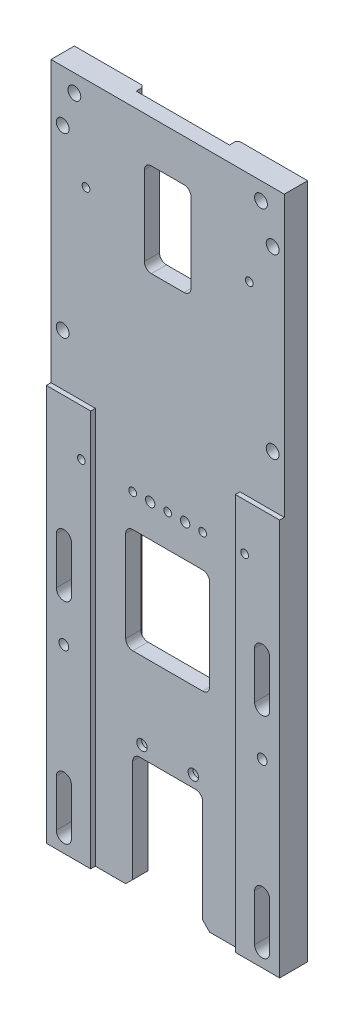
from build123d import *

# Parameters (mm, degrees)
SKETCH1_W                                            = 100
SKETCH1_H                                            = 290
BOSS_EXTRUDE1_DEPTH                                  = 10
SKETCH4_W                                            = 40
SKETCH4_H                                            = 290
CUT_EXTRUDE3_DEPTH                                   = 3.5
SKETCH5_R                                            = 2.75
CUT_EXTRUDE4_DEPTH                                   = 18
LPATTERN1_COUNT                                      = 2
LPATTERN1_PITCH                                      = 76
CUT_EXTRUDE5_DEPTH                                   = 18
LPATTERN2_COUNT                                      = 2
LPATTERN2_PITCH                                      = 90
SKETCH9_W                                            = 30
SKETCH9_H                                            = 50
CUT_EXTRUDE7_DEPTH                                   = 25
BOSS_EXTRUDE3_START                                  = 2
SKETCH11_W                                           = 19
SKETCH11_H                                           = 170
BOSS_EXTRUDE3_DEPTH                                  = 2
SKETCH12_R                                           = 2.75
CUT_EXTRUDE8_DEPTH                                   = 154.704261489
CHAMFER1_SIZE                                        = 3
FILLET1_R                                            = 3
SKETCH20_R                                           = 2
CUT_EXTRUDE14_DEPTH                                  = 10
M5_TAPPED_HOLE1_D                                    = 4.2
M4_TAPPED_HOLE2_D                                    = 3.3
F_4_0_4_DIAMETER_HOLE1_D                             = 4
CUT_EXTRUDE15_DEPTH                                  = 154.704261489
CHAMFER2_SIZE                                        = 1
HOLE_SIZE_PER_SOCKET_HEAD_CAP_SCREW_TYPE_D           = 4.5
HOLE_SIZE_PER_SOCKET_HEAD_CAP_SCREW_TYPE_CBORE_D     = 8
HOLE_SIZE_PER_SOCKET_HEAD_CAP_SCREW_TYPE_CBORE_DEPTH = 4.5
CUT_EXTRUDE16_DEPTH                                  = 154.847326919
M4_TAPPED_HOLE4_D                                    = 3.3


with BuildPart() as part:
    # Sketch1 → Boss-Extrude1 (new body)
    with BuildSketch(Plane.XY):
        Rectangle(SKETCH1_W, SKETCH1_H)
    extrude(amount=BOSS_EXTRUDE1_DEPTH)

    # Sketch4 → Cut-Extrude3 (cut)
    with BuildSketch(Plane(origin=(0, 0, 0), x_dir=(-1, 0, 0), z_dir=(0, 0, -1))):
        Rectangle(SKETCH4_W, SKETCH4_H)
    extrude(amount=-CUT_EXTRUDE3_DEPTH, mode=Mode.SUBTRACT)

    # Sketch5 → Cut-Extrude4 (cut)
    with BuildSketch(Plane.XY.offset(10)):
        with Locations((-45, 123)):
            Circle(SKETCH5_R)
        with Locations((45, 123)):
            Circle(SKETCH5_R)
    cut_extrude4 = extrude(amount=-CUT_EXTRUDE4_DEPTH, mode=Mode.SUBTRACT)

    # LPattern1: Cut-Extrude4 ×2
    with Locations(*[(0, -i * LPATTERN1_PITCH, 0) for i in range(1, LPATTERN1_COUNT)]):
        add(cut_extrude4, mode=Mode.SUBTRACT)

    # Sketch6 → Cut-Extrude5 (cut)
    with BuildSketch(Plane.XY.offset(10)):
        with BuildLine():
            Line((-39.25, -28), (-39.25, -48))
            ThreePointArc((-39.25, -48), (-42.5, -51.25), (-45.75, -48))
            Line((-45.75, -48), (-45.75, -28))
            ThreePointArc((-45.75, -28), (-42.5, -24.75), (-39.25, -28))
        make_face()
        with BuildLine():
            Line((39.25, -28), (39.25, -48))
            ThreePointArc((39.25, -48), (42.5, -51.25), (45.75, -48))
            Line((45.75, -48), (45.75, -28))
            ThreePointArc((45.75, -28), (42.5, -24.75), (39.25, -28))
        make_face()
    cut_extrude5 = extrude(amount=-CUT_EXTRUDE5_DEPTH, mode=Mode.SUBTRACT)

    # LPattern2: Cut-Extrude5 ×2
    with Locations(*[(0, -i * LPATTERN2_PITCH, 0) for i in range(1, LPATTERN2_COUNT)]):
        add(cut_extrude5, mode=Mode.SUBTRACT)

    # Sketch9 → Cut-Extrude7 (cut)
    with BuildSketch(Plane.XY.offset(10)):
        with Locations((0, -120)):
            Rectangle(SKETCH9_W, SKETCH9_H)
    extrude(amount=-CUT_EXTRUDE7_DEPTH, mode=Mode.SUBTRACT)

    # Sketch11 → Boss-Extrude3 (add)
    # profile 1 of 2: a face of its own
    with BuildSketch(Plane.XY.offset(10).offset(BOSS_EXTRUDE3_START)):
        with Locations((-40.5, -60)):
            Rectangle(SKETCH11_W, SKETCH11_H)
        with BuildLine():
            Line((-39.25, -138), (-39.25, -118))
            ThreePointArc((-39.25, -118), (-42.5, -114.75), (-45.75, -118))
            Line((-45.75, -118), (-45.75, -138))
            ThreePointArc((-45.75, -138), (-42.5, -141.25), (-39.25, -138))
        make_face(mode=Mode.SUBTRACT)
        with BuildLine():
            Line((-39.25, -48), (-39.25, -28))
            ThreePointArc((-39.25, -28), (-42.5, -24.75), (-45.75, -28))
            Line((-45.75, -28), (-45.75, -48))
            ThreePointArc((-45.75, -48), (-42.5, -51.25), (-39.25, -48))
        make_face(mode=Mode.SUBTRACT)
    # profile 2 of 2: a face of its own
    with BuildSketch(Plane.XY.offset(10).offset(BOSS_EXTRUDE3_START)):
        with Locations((40.5, -60)):
            Rectangle(SKETCH11_W, SKETCH11_H)
        with BuildLine():
            Line((45.75, -138), (45.75, -118))
            ThreePointArc((45.75, -118), (42.5, -114.75), (39.25, -118))
            Line((39.25, -118), (39.25, -138))
            ThreePointArc((39.25, -138), (42.5, -141.25), (45.75, -138))
        make_face(mode=Mode.SUBTRACT)
        with BuildLine():
            Line((45.75, -48), (45.75, -28))
            ThreePointArc((45.75, -28), (42.5, -24.75), (39.25, -28))
            Line((39.25, -28), (39.25, -48))
            ThreePointArc((39.25, -48), (42.5, -51.25), (45.75, -48))
        make_face(mode=Mode.SUBTRACT)
    extrude(amount=-BOSS_EXTRUDE3_DEPTH)

    # Sketch12 → Cut-Extrude8 (cut, through all)
    with BuildSketch(Plane.XY.offset(10)):
        with Locations((-40, 137.5)):
            Circle(SKETCH12_R)
        with Locations(Location((40, 137.5, 0), (0, 0, 180))):
            Circle(SKETCH12_R)
    extrude(amount=-CUT_EXTRUDE8_DEPTH, mode=Mode.SUBTRACT)

    # Chamfer1
    chamfer1_edges = [part.edges().sort_by_distance(p)[0] for p in [
        (15, -145, 6.75),
        (-15, -145, 6.75),
    ]]
    chamfer(chamfer1_edges, length=CHAMFER1_SIZE)

    # Fillet1
    fillet1_edges = [part.edges().sort_by_distance(p)[0] for p in [
        (15, -95, 6.75),
        (-15, -95, 6.75),
    ]]
    fillet(fillet1_edges, radius=FILLET1_R)

    # Sketch20 → Cut-Extrude14 (cut)
    with BuildSketch(Plane.XY.offset(12)):
        with Locations((-42.5, -67.5)):
            Circle(SKETCH20_R)
        with Locations(Location((42.5, -67.5, 0), (0, 0, 180))):
            Circle(SKETCH20_R)
    extrude(amount=-CUT_EXTRUDE14_DEPTH, mode=Mode.SUBTRACT)

    # M5 Tapped Hole1 (through all)
    with Locations(Plane(origin=(-42.5, -67.5, 12), x_dir=(1, 0, 0), z_dir=(0, 0, 1))):
        with Locations((0, 0), (85, 0)):
            Hole(M5_TAPPED_HOLE1_D / 2)

    # M4 Tapped Hole2 (through all)
    with Locations(Plane.XY.offset(10)):
        with Locations((-15, 2), (0, 2), (15, 2)):
            Hole(M4_TAPPED_HOLE2_D / 2)

    # Ø4.0 (4) Diameter Hole1 (through all)
    with Locations(Plane.XY.offset(10)):
        with Locations((-7.5, 2), (7.5, 2)):
            Hole(F_4_0_4_DIAMETER_HOLE1_D / 2)

    # Sketch26 → Cut-Extrude15 (cut, through all)
    with BuildSketch(Plane.XY.offset(10)):
        with BuildLine():
            Line((-7, 127), (7, 127))
            ThreePointArc((7, 127), (9.121320344, 126.121320344), (10, 124))
            Line((10, 124), (10, 90))
            ThreePointArc((10, 90), (9.121320344, 87.878679656), (7, 87))
            Line((7, 87), (-7, 87))
            ThreePointArc((-7, 87), (-9.121320344, 87.878679656), (-10, 90))
            Line((-10, 90), (-10, 124))
            ThreePointArc((-10, 124), (-9.121320344, 126.121320344), (-7, 127))
        make_face()
    extrude(amount=-CUT_EXTRUDE15_DEPTH, mode=Mode.SUBTRACT)

    # Chamfer2
    chamfer2_edges = [part.edges().sort_by_distance(p)[0] for p in [
        (20, 0, 0),
        (-20, 0, 0),
    ]]
    chamfer(chamfer2_edges, length=CHAMFER2_SIZE)

    # Hole size per socket head cap screw type1 (through all)
    with Locations(Plane(origin=(0, 0, 3.5), x_dir=(-1, 0, 0), z_dir=(0, 0, -1))):
        with Locations((-11, -90), (11, -90)):
            CounterBoreHole(HOLE_SIZE_PER_SOCKET_HEAD_CAP_SCREW_TYPE_D / 2, HOLE_SIZE_PER_SOCKET_HEAD_CAP_SCREW_TYPE_CBORE_D / 2, HOLE_SIZE_PER_SOCKET_HEAD_CAP_SCREW_TYPE_CBORE_DEPTH)

    # Sketch31 → Cut-Extrude16 (cut, through all)
    with BuildSketch(Plane.XY.offset(12)):
        with BuildLine():
            Line((-15, -12), (15, -12))
            ThreePointArc((15, -12), (17.121320344, -12.878679656), (18, -15))
            Line((18, -15), (18, -54))
            ThreePointArc((18, -54), (17.121320344, -56.121320344), (15, -57))
            Line((15, -57), (-15, -57))
            ThreePointArc((-15, -57), (-17.121320344, -56.121320344), (-18, -54))
            Line((-18, -54), (-18, -15))
            ThreePointArc((-18, -15), (-17.121320344, -12.878679656), (-15, -12))
        make_face()
    extrude(amount=-CUT_EXTRUDE16_DEPTH, mode=Mode.SUBTRACT)

    # M4 Tapped Hole4 (through all)
    with Locations(Plane(origin=(0, 0, 0), x_dir=(-1, 0, 0), z_dir=(0, 0, -1))):
        with Locations((-35, 105), (35, 105), (35, 5), (-35, 5)):
            Hole(M4_TAPPED_HOLE4_D / 2)


solid = part.part
